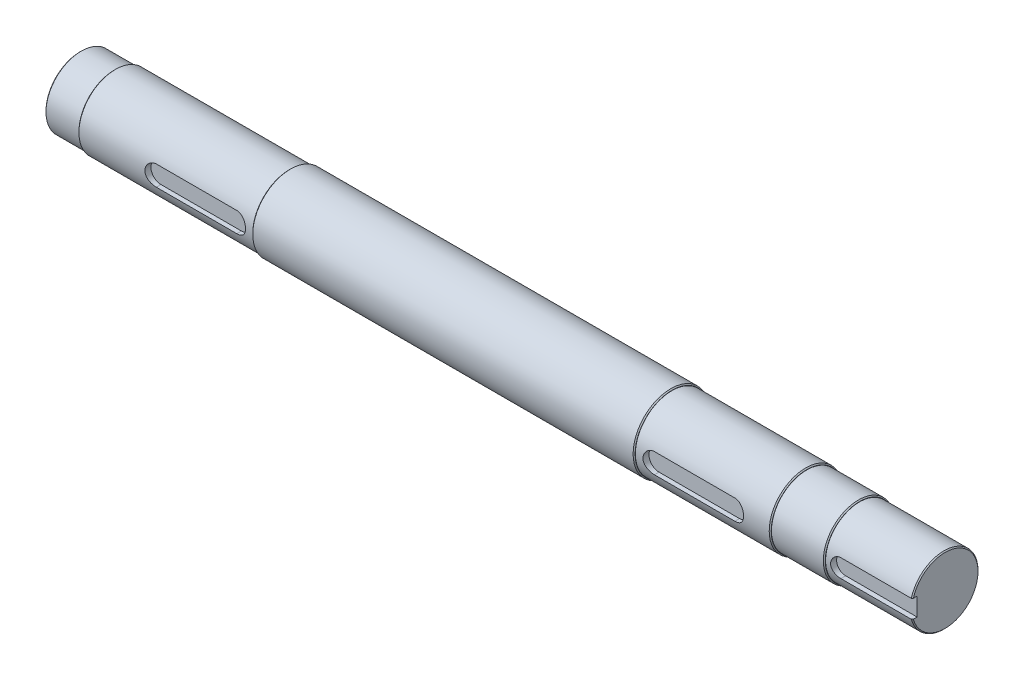
SolidWorks part; units mm, degrees
material "热轧圆钢 45"
ref_plane "Front Plane" through (0, 0, 0) normal (0, 0, 1) x (1, 0, 0)
ref_plane "Top Plane" through (0, 0, 0) normal (0, 1, 0) x (1, 0, 0)
ref_plane "Right Plane" through (0, 0, 0) normal (1, 0, 0) x (0, 0, -1)
sketch "Sketch1" plane through (0, 0, 0) normal (0, 0, 1) x (1, 0, 0)
  line L0 (-820.6626, 0) -> (1121.6597, 0) construction
  line L1 (0, 78) -> (0, 0) construction
  line L3 (923, 18) -> (781, 18) construction
  line L4 (923, -18) -> (781, -18) construction
  line L5 (923, 0) -> (923, 18) construction
  line L6 (-575, 20) -> (-415, 20) construction
  line L7 (-575, -20) -> (-415, -20) construction
  line L9 (-796, 70) -> (-728, 70)
  line L10 (-796, 0) -> (923, 0)
  line L11 (-796, 70) -> (-796, 0)
  line L12 (923, 0) -> (923, -18) construction
  line L15 (-728, 72.5) -> (-380, 72.5)
  line L17 (-728, 72.5) -> (-728, 70)
  line L21 (-380, 75) -> (-380, 72.5)
  line L25 (-380, 75) -> (380, 75)
  line L27 (380, 75) -> (380, 72.5)
  line L31 (380, 72.5) -> (648, 72.5)
  line L33 (648, 72.5) -> (648, 70)
  line L37 (648, 70) -> (753, 70)
  line L39 (753, 70) -> (753, 67.5)
  line L43 (753, 67.5) -> (923, 67.5)
  line L45 (923, 67.5) -> (923, 0)
  arc A0 (781, 18) -> (781, -18) centre (781, 0) ccw construction
  arc A1 (-575, 20) -> (-575, -20) centre (-575, 0) ccw construction
  arc A2 (-415, -20) -> (-415, 20) centre (-415, 0) ccw construction
  dimension "D17" = 35
  dimension "D13" = 160
  dimension "D1" = 140
  dimension "D2" = 68
  dimension "D3" = 145
  dimension "D4" = 348
  dimension "D5" = 760
  dimension "D6" = 150
  dimension "D7" = 268
  dimension "D8" = 145
  dimension "D9" = 140
  dimension "D10" = 105
  dimension "D11" = 135
  dimension "D12" = 170
  dimension "D14" = 36
  dimension "D15" = 160
  dimension "D16" = 40
revolve "Revolve1" add sketch "Sketch1" angle 360 about L0
ref_plane "Plane2" through (0, 0, 67.5) normal (0, 0, 1) x (1, 0, 0)
sketch "Sketch2" plane through (0, 0, 67.5) normal (0, 0, 1) x (1, 0, 0)
  line L0 (923, -18) -> (781, -18) construction
  line L1 (923, -18) -> (781, -18)
  line L2 (923, 18) -> (781, 18) construction
  line L3 (923, 0) -> (923, -18) construction
  line L4 (923, 67.5) -> (923, 0) construction
  line L5 (923, 18) -> (781, 18)
  line L6 (923, 0) -> (923, -18)
  line L7 (923, 18) -> (923, 0)
  arc A0 (781, 18) -> (781, -18) centre (781, 0) ccw construction
  arc A1 (781, 18) -> (781, -18) centre (781, 0) ccw
extrude "Cut-Extrude1" cut sketch "Sketch2" against normal blind 12
ref_plane "Plane3" through (0, 0, 72.5) normal (0, 0, 1) x (1, 0, 0)
sketch "Sketch3" plane through (0, 0, 72.5) normal (0, 0, 1) x (1, 0, 0)
  line L0 (-575, -20) -> (-415, -20) construction
  line L1 (-575, -20) -> (-415, -20)
  line L2 (-575, 20) -> (-415, 20) construction
  line L3 (-575, 20) -> (-415, 20)
  line L4 (0, 0) -> (0, -209.4009) construction
  line L5 (575, 20) -> (415, 20)
  line L6 (575, -20) -> (415, -20)
  arc A0 (-575, 20) -> (-575, -20) centre (-575, 0) ccw construction
  arc A1 (-415, -20) -> (-415, 20) centre (-415, 0) ccw construction
  arc A2 (-575, 20) -> (-575, -20) centre (-575, 0) ccw
  arc A3 (-415, -20) -> (-415, 20) centre (-415, 0) ccw
  arc A4 (415, -20) -> (415, 20) centre (415, 0) cw
  arc A5 (575, 20) -> (575, -20) centre (575, 0) cw
extrude "Cut-Extrude2" cut sketch "Sketch3" against normal blind 12
chamfer "Chamfer1" distance 2 angle 45 7 edges at (923, 0, -67.5) (753, 0, 70) (648, 0, 72.5) (380, 0, 75) (-380, 0, 75) (-728, 0, 72.5) (-796, 0, 70)
